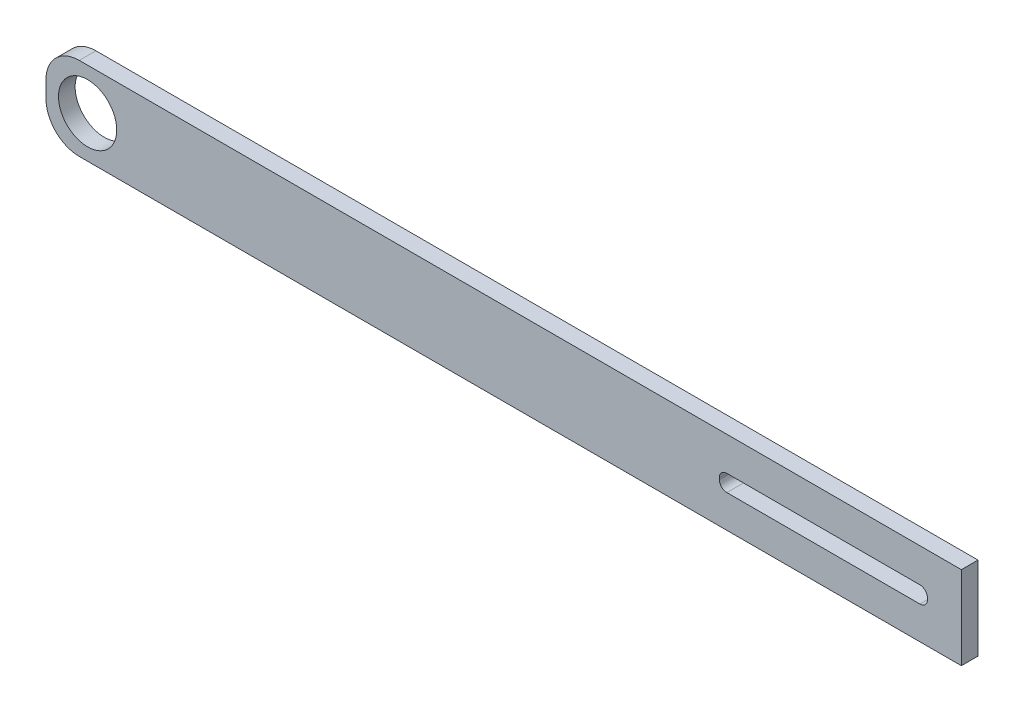
SolidWorks part; units mm, degrees
material "PVC Rigid"
ref_plane "Front Plane" through (0, 0, 0) normal (0, 0, 1) x (1, 0, 0)
ref_plane "Top Plane" through (0, 0, 0) normal (0, 1, 0) x (1, 0, 0)
ref_plane "Right Plane" through (0, 0, 0) normal (1, 0, 0) x (0, 0, -1)
sketch "Sketch1" plane through (0, 0, 0) normal (0, 0, 1) x (1, 0, 0)
  line L1 (275, -25) -> (-275, -25)
  line L2 (275, -25) -> (275, 25)
  line L3 (275, 25) -> (-275, 25)
  line L4 (-275, -25) -> (-275, 25)
  line L5 (275, -25) -> (-275, 25) construction
  line L6 (275, 25) -> (-275, -25) construction
  point P0 (0, 0)
  dimension "D1" = 50
  dimension "D2" = 550
extrude "Boss-Extrude1" add sketch "Sketch1" along normal blind 10
sketch "Sketch2" plane through (0, 0, 10) normal (0, 0, 1) x (1, 0, 0)
  line L0 (-260.8215, 0) -> (-183.8915, 0) construction
  line L1 (-275, 25) -> (-225, -25) construction
  line L2 (-275, -25) -> (275, -25) construction
  line L3 (-275, 25) -> (-275, -25) construction
  circle A0 centre (-250, 0) radius 17.5
  dimension "D2" = 35
  dimension "D1" = 45
extrude "Cut-Extrude1" cut sketch "Sketch2" against normal blind 10
sketch "Sketch3" plane through (0, 0, 10) normal (0, 0, 1) x (1, 0, 0)
  line L1 (250.0998, -5.341) -> (134.0998, -5.341)
  line L2 (254.5998, -0.841) -> (254.5998, 0.159)
  line L3 (250.0998, 4.659) -> (134.0998, 4.659)
  line L4 (129.5998, -0.841) -> (129.5998, 0.159)
  line L5 (254.5998, -5.341) -> (129.5998, 4.659) construction
  line L6 (254.5998, 4.659) -> (129.5998, -5.341) construction
  arc A0 (250.0998, -5.341) -> (254.5998, -0.841) centre (250.0998, -0.841) ccw
  arc A1 (254.5998, 0.159) -> (250.0998, 4.659) centre (250.0998, 0.159) ccw
  arc A2 (134.0998, -5.341) -> (129.5998, -0.841) centre (134.0998, -0.841) cw
  arc A3 (134.0998, 4.659) -> (129.5998, 0.159) centre (134.0998, 0.159) ccw
  point P0 (192.0998, -0.341)
  dimension "D3" = 4.5
  dimension "D1" = 125
  dimension "D2" = 10
extrude "Cut-Extrude2" cut sketch "Sketch3" against normal blind 10
fillet "Fillet1" radius 20 2 edges at (-275, -25, 5) (-275, 25, 5)
